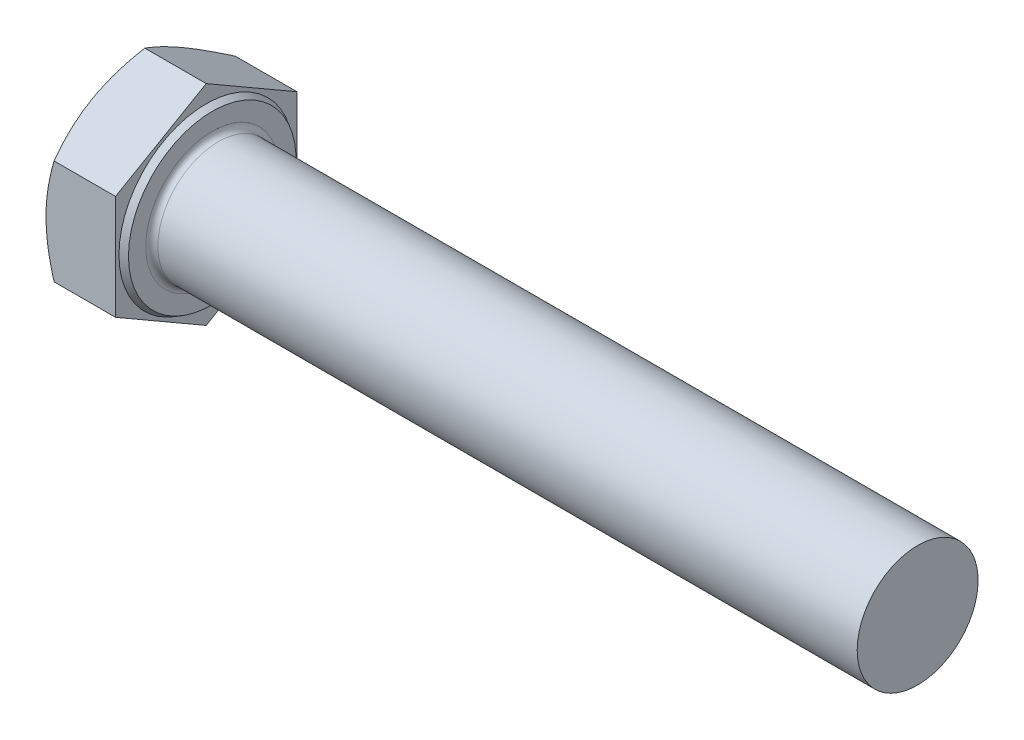
from build123d import *

# Parameters (mm, degrees)
BASE_EXTRUDE_DEPTH = 7.5
FILLET_2_R         = 0.6


with BuildPart() as part:
    # Sketch1 → Base-Extrude (new body)
    with BuildSketch(Plane(origin=(0, 0, 0), x_dir=(0, 0, -1), z_dir=(1, 0, 0))):
        Polygon((9, 5.196152423), (9, -5.196152423), (0, -10.392304845), (-9, -5.196152423), (-9, 5.196152423), (0, 10.392304845), align=None)
    extrude(amount=BASE_EXTRUDE_DEPTH)

    # Sketch2 → Boss-Revolve1 (revolve)
    with BuildSketch(Plane.XY, mode=Mode.PRIVATE) as boss_revolve1_sk:
        Polygon((0, 0), (77.5, 0), (77.5, 4.4845), (77.5, 6), (47.5, 6), (0, 6), align=None)
    revolve(boss_revolve1_sk.sketch.rotate(Axis((0, 0, 0), (1, 0, 0)), 90), axis=Axis((0, 0, 0), (1, 0, 0)))

    # Sketch3 → Cut-Revolve1 (revolve, cut)
    with BuildSketch(Plane.XY):
        Polygon((0, 9), (3.690598923, 15.392304845), (3.690598923, 20.392304845), (-10, 20.392304845), (-10, 9), align=None)
    revolve(axis=Axis((0, 0, 0), (1, 0, 0)), mode=Mode.SUBTRACT)

    # Sketch4 → Cut-Revolve3 (revolve, cut)
    with BuildSketch(Plane.XY, mode=Mode.PRIVATE) as cut_revolve3_sk:
        Polygon((7.5, 8.315), (6.9, 8.661410162), (6.9, 10.392304845), (7.5, 10.392304845), align=None)
    revolve(cut_revolve3_sk.sketch.rotate(Axis((0, 0, 0), (1, 0, 0)), 90), axis=Axis((0, 0, 0), (1, 0, 0)), mode=Mode.SUBTRACT)

    # Fillet 2
    fillet_2_edges = [part.edges().sort_by_distance(p)[0] for p in [
        (7.5, 0, -6),
    ]]
    fillet(fillet_2_edges, radius=FILLET_2_R)


solid = part.part
